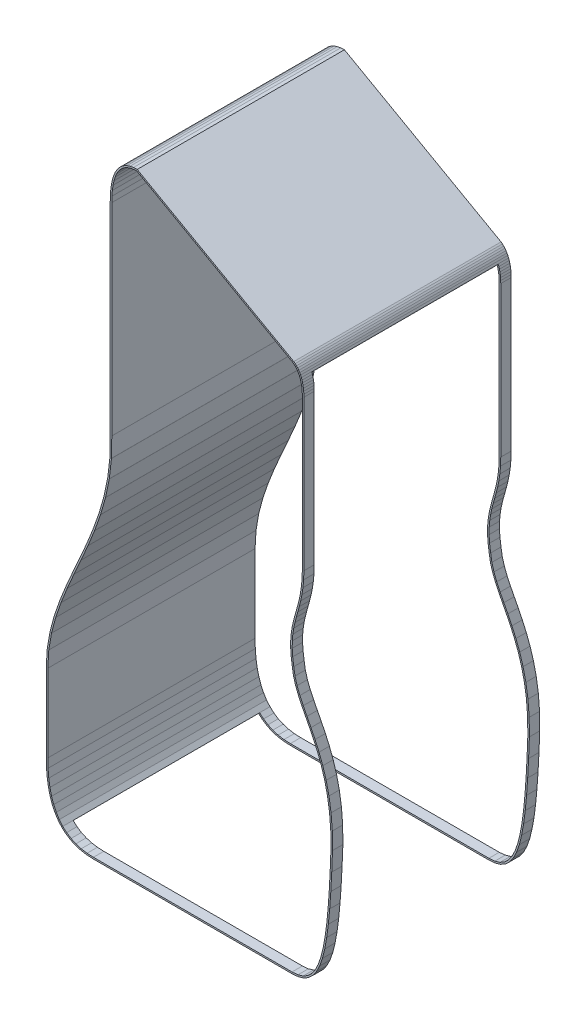
from build123d import *

# Parameters (mm, degrees)
EXTRUDE_1_DEPTH     = 200
SKETCH_2_W          = 180
SKETCH_2_H          = 1020
CUT_EXTRUDE_1_DEPTH = 180
SKETCH_3_W          = 700
SKETCH_3_H          = 40
CUT_EXTRUDE_2_DEPTH = 180


with BuildPart() as part:
    # 草图1 → 凸台-拉伸1 (new, symmetric)
    with BuildSketch(Plane.XY):
        Polygon((103, 235), (-24.833333333, 235), (-152.666666667, 235), (-280.5, 235), (-293.035714286, 235.637755102), (-304.642857143, 237.551020408), (-315.321428571, 240.739795918), (-325.071428571, 245.204081633), (-333.892857143, 250.943877551), (-341.785714286, 257.959183673), (-348.75, 266.25), (-354.785714286, 275.816326531), (-359.892857143, 286.658163265), (-364.071428571, 298.775510204), (-367.321428571, 312.168367347), (-369.642857143, 326.836734694), (-371.035714286, 342.780612245), (-371.5, 360), (-371.5, 410), (-371.5, 460), (-371.5, 510), (-369.607325073, 541.716472303), (-364.317784257, 572.711370262), (-356.214103499, 603.18148688), (-345.879008746, 633.32361516), (-333.895225948, 663.334548105), (-320.84548105, 693.411078717), (-307.3125, 723.75), (-293.879008746, 754.548104956), (-281.127733236, 786.002186589), (-269.641399417, 818.309037901), (-260.002733236, 851.665451895), (-252.794460641, 886.268221574), (-248.59930758, 922.314139942), (-248, 960), (-248, 1090), (-248, 1220), (-248, 1350), (-247.734693878, 1361.020408163), (-246.93877551, 1371.224489796), (-245.612244898, 1380.612244898), (-243.755102041, 1389.183673469), (-241.367346939, 1396.93877551), (-238.448979592, 1403.87755102), (-235, 1410), (-231.020408163, 1415.306122449), (-226.510204082, 1419.795918367), (-221.469387755, 1423.469387755), (-215.897959184, 1426.326530612), (-209.795918367, 1428.367346939), (-203.163265306, 1429.591836735), (-196, 1430), (-95.25, 1373.333333333), (5.5, 1316.666666667), (106.25, 1260), (108.93622449, 1257.887755102), (111.423469388, 1255.551020408), (113.711734694, 1252.989795918), (115.801020408, 1250.204081633), (117.691326531, 1247.193877551), (119.382653061, 1243.959183673), (120.875, 1240.5), (122.168367347, 1236.816326531), (123.262755102, 1232.908163265), (124.158163265, 1228.775510204), (124.854591837, 1224.418367347), (125.352040816, 1219.836734694), (125.650510204, 1215.030612245), (125.75, 1210), (125.75, 1113.333333333), (125.75, 1016.666666667), (125.75, 920), (125.280976676, 904.7303207), (123.987609329, 890.903790087), (122.040451895, 878.279883382), (119.610058309, 866.618075802), (116.866982507, 855.677842566), (113.981778426, 845.218658892), (111.125, 835), (108.467201166, 824.781341108), (106.17893586, 814.322157434), (104.430758017, 803.381924198), (103.393221574, 791.720116618), (103.236880466, 779.096209913), (104.13228863, 765.2696793), (106.25, 750), (108.586825802, 735.40451895), (112.60787172, 721.39941691), (118.007561953, 707.656705539), (124.4803207, 693.848396501), (131.720572157, 679.646501458), (139.422740525, 664.72303207), (147.28125, 648.75), (154.990524781, 631.39941691), (162.244989067, 612.343294461), (168.739067055, 591.253644315), (174.167182945, 567.802478134), (178.223760933, 541.66180758), (180.603225219, 512.503644315), (181, 480), (179.493440233, 443.170553936), (177.702623907, 409.752186589), (175.542274052, 379.635568513), (172.927113703, 352.711370262), (169.771865889, 328.870262391), (165.991253644, 308.002915452), (161.5, 290), (156.212827988, 274.752186589), (150.044460641, 262.150145773), (142.909620991, 252.084548105), (134.72303207, 244.44606414), (125.39941691, 239.125364431), (114.853498542, 236.013119534), align=None)
        Polygon((102.872028159, 238), (-280.423736739, 238), (-292.714523775, 238.625294416), (-303.966988146, 240.480096235), (-314.262647627, 243.554528713), (-323.621022127, 247.839498722), (-332.068073639, 253.335700544), (-339.629257794, 260.056210055), (-346.321660401, 268.023356015), (-352.150234117, 277.261374374), (-357.109690944, 287.789691813), (-361.189318319, 299.620113078), (-364.377334557, 312.75754263), (-366.663357931, 327.202195816), (-368.039238085, 342.951739712), (-368.5, 360.040437096), (-368.5, 509.910567311), (-366.622439806, 541.373754696), (-361.383494487, 572.072180363), (-353.342030058, 602.30836146), (-343.065324819, 632.280197715), (-331.125524275, 662.180986098), (-318.099458424, 692.202942191), (-304.572710651, 722.527889398), (-304.562695939, 722.550592801), (-291.129204686, 753.348697757), (-291.098779272, 753.421018417), (-278.347503761, 784.87510005), (-278.301074069, 784.997200047), (-266.814740249, 817.304051359), (-266.759311447, 817.476230038), (-257.120645267, 850.832644032), (-257.065781169, 851.053641011), (-249.857508575, 885.656410691), (-249.814574246, 885.921411725), (-245.619421185, 921.967330092), (-245.599686853, 922.266437821), (-245.000379273, 959.952297879), (-245, 960), (-245, 1349.96389412), (-244.737504548, 1360.867551339), (-243.955156614, 1370.897653056), (-242.657080202, 1380.084039978), (-240.850247739, 1388.423266731), (-238.544103314, 1395.913308452), (-235.750503648, 1402.555433532), (-232.48240216, 1408.35679712), (-228.750381511, 1413.332824652), (-224.557063902, 1417.507167973), (-219.891921874, 1420.906866617), (-214.731067969, 1423.553458363), (-209.044140566, 1425.455440772), (-202.804197237, 1426.60743031), (-196.705651059, 1426.954925819), (-96.720681035, 1370.718548965), (104.577586437, 1257.49867975), (106.978203447, 1255.611015092), (109.273707528, 1253.454418438), (111.388885082, 1251.086928735), (113.32648331, 1248.503464431), (115.087710102, 1245.698811779), (116.672340705, 1242.668175875), (118.07901936, 1239.407566889), (119.305644973, 1235.913982302), (120.34974247, 1232.185410357), (121.208760086, 1228.220713665), (121.880272699, 1224.019455268), (122.362098627, 1219.581714926), (122.65234996, 1214.907924237), (122.75, 1209.970337586), (122.75, 920.046063123), (122.28527307, 904.91625863), (121.009001201, 891.272484413), (119.087505078, 878.814946384), (116.685464961, 867.289187834), (113.965627687, 856.441637022), (111.091168693, 846.021405482), (108.235781783, 835.807724023), (108.221598055, 835.755153723), (105.563799221, 825.536494831), (105.536519768, 825.422517014), (103.248254462, 814.96333334), (103.216518576, 814.795532375), (101.468340733, 803.855299139), (101.442561151, 803.647780338), (100.405024708, 791.985972758), (100.393451613, 791.757267349), (100.237110505, 779.133360643), (100.243151563, 778.902335587), (101.138559727, 765.075804975), (101.160730264, 764.857561743), (103.278441635, 749.587882442), (103.28772716, 749.525721997), (105.624552962, 734.930240948), (105.70332169, 734.576627629), (109.724367609, 720.571525588), (109.815670342, 720.302324633), (115.215360575, 706.559613262), (115.291193755, 706.383385543), (121.763952502, 692.575076505), (121.807607564, 692.485823752), (129.047859022, 678.283928709), (129.054690715, 678.270610424), (136.743624445, 663.372784037), (144.563505547, 647.478267142), (152.215841458, 630.255831333), (159.406560727, 611.367155133), (165.840451771, 590.472963314), (171.219580971, 567.233435022), (175.242553169, 541.309320858), (177.604716559, 512.363164274), (177.999251226, 480.043029363), (176.49672283, 443.312134431), (174.708372871, 409.939791881), (172.552669263, 379.887945366), (169.946206065, 353.053288023), (166.807177673, 329.334734389), (163.05676512, 308.634076704), (158.62165463, 290.856207652), (153.438131207, 275.907309114), (147.456622699, 263.687022914), (140.639163297, 254.069174886), (132.932228181, 246.878231153), (124.215581525, 241.903909656), (114.295534992, 238.976368105), align=None, mode=Mode.SUBTRACT)
    extrude(amount=EXTRUDE_1_DEPTH, both=True)

    # 草图2 → 切除-拉伸1 (cut, symmetric)
    with BuildSketch(Plane.XY):
        with Locations((150, 730)):
            Rectangle(SKETCH_2_W, SKETCH_2_H)
    extrude(amount=CUT_EXTRUDE_1_DEPTH, both=True, mode=Mode.SUBTRACT)

    # 草图3 → 切除-拉伸2 (cut, symmetric)
    with BuildSketch(Plane.XY):
        with Locations((-250, 240)):
            Rectangle(SKETCH_3_W, SKETCH_3_H)
    extrude(amount=CUT_EXTRUDE_2_DEPTH, both=True, mode=Mode.SUBTRACT)


solid = part.part
